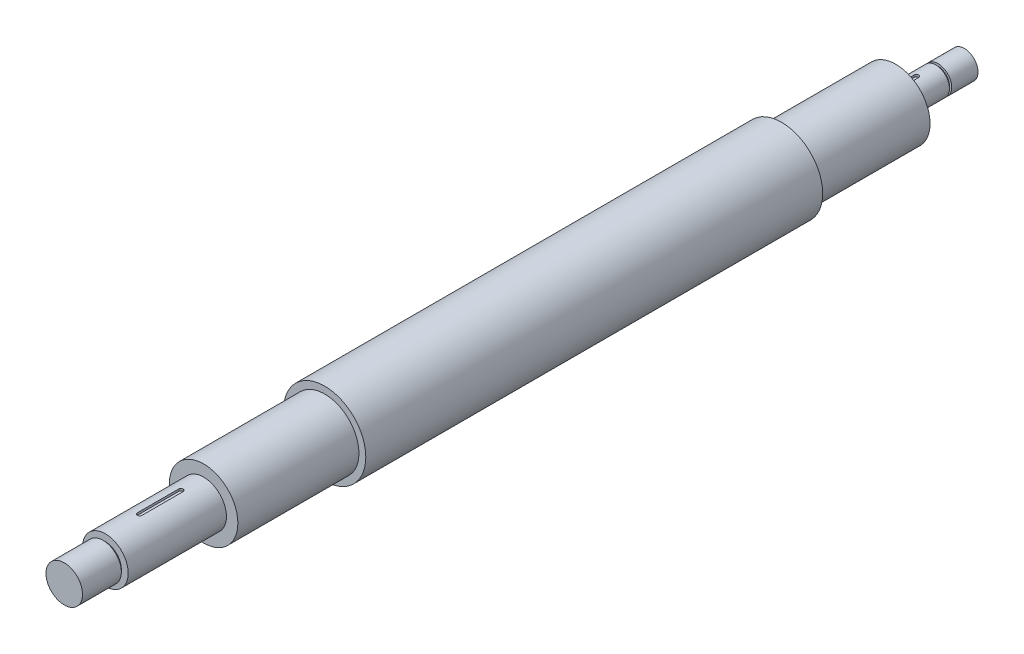
from build123d import *

# Parameters (mm, degrees)
SKETCH1_R           = 15
BOSS_EXTRUDE1_DEPTH = 50
SKETCH2_R           = 18
BOSS_EXTRUDE2_DEPTH = 200
SKETCH3_R           = 15
BOSS_EXTRUDE3_DEPTH = 53
SKETCH4_R           = 6
BOSS_EXTRUDE4_DEPTH = 30
CUT_EXTRUDE1_START  = 5
CUT_EXTRUDE1_DEPTH  = 10
CUT_EXTRUDE3_START  = -12.5
SKETCH6_R           = 6
SKETCH6_R_2         = 5
CUT_EXTRUDE3_DEPTH  = 1
SKETCH7_R           = 10
BOSS_EXTRUDE5_DEPTH = 43
CUT_EXTRUDE4_START  = 4
CUT_EXTRUDE4_DEPTH  = 12
SKETCH8_R           = 8
BOSS_EXTRUDE6_DEPTH = 18
CUT_EXTRUDE6_START  = -18
SKETCH10_R          = 9
SKETCH10_R_2        = 7
CUT_EXTRUDE6_DEPTH  = 1


with BuildPart() as part:
    # Sketch1 → Boss-Extrude1 (new body)
    with BuildSketch(Plane.XY):
        Circle(SKETCH1_R)
    extrude(amount=BOSS_EXTRUDE1_DEPTH)

    # Sketch2 → Boss-Extrude2 (add)
    with BuildSketch(Plane.XY.offset(50)):
        Circle(SKETCH2_R)
    extrude(amount=BOSS_EXTRUDE2_DEPTH)

    # Sketch3 → Boss-Extrude3 (add)
    with BuildSketch(Plane.XY.offset(250)):
        Circle(SKETCH3_R)
    extrude(amount=BOSS_EXTRUDE3_DEPTH)

    # Sketch4 → Boss-Extrude4 (add)
    with BuildSketch(Plane(origin=(0, 0, 0), x_dir=(-1, 0, 0), z_dir=(0, 0, -1))):
        with Locations(Location((0, 0, 0), (0, 0, 180))):
            Circle(SKETCH4_R)
    extrude(amount=BOSS_EXTRUDE4_DEPTH)

    # Sketch5 → Cut-Extrude1 (cut)
    with BuildSketch(Plane(origin=(0, 0, 0), x_dir=(1, 0, 0), z_dir=(0, 1, 0)).offset(CUT_EXTRUDE1_START)):
        with BuildLine():
            ThreePointArc((-1, 9), (0, 8), (1, 9))
            Line((1, 9), (-1, 9))
        make_face()
        with BuildLine():
            Line((-1, 9), (1, 9))
            ThreePointArc((1, 9), (0, 10), (-1, 9))
        make_face()
        with BuildLine():
            Line((1, 5), (1, 9))
            ThreePointArc((1, 9), (0, 8), (-1, 9))
            Line((-1, 9), (-1, 5))
            ThreePointArc((-1, 5), (0, 6), (1, 5))
        make_face()
        with BuildLine():
            ThreePointArc((-1, 5), (0, 4), (1, 5))
            Line((1, 5), (-1, 5))
        make_face()
        with BuildLine():
            Line((-1, 5), (1, 5))
            ThreePointArc((1, 5), (0, 6), (-1, 5))
        make_face()
    extrude(amount=CUT_EXTRUDE1_DEPTH, mode=Mode.SUBTRACT)

    # Sketch6 → Cut-Extrude3 (cut)
    with BuildSketch(Plane(origin=(0, 0, -30), x_dir=(-1, 0, 0), z_dir=(0, 0, -1)).offset(CUT_EXTRUDE3_START)):
        with Locations(Location((0, 0, 0), (0, 0, 180))):
            Circle(SKETCH6_R)
        Circle(SKETCH6_R_2, mode=Mode.SUBTRACT)
    extrude(amount=CUT_EXTRUDE3_DEPTH, mode=Mode.SUBTRACT)

    # Sketch7 → Boss-Extrude5 (add)
    with BuildSketch(Plane.XY.offset(303)):
        Circle(SKETCH7_R)
    extrude(amount=BOSS_EXTRUDE5_DEPTH)

    # Sketch9 → Cut-Extrude4 (cut)
    with BuildSketch(Plane(origin=(0, 5, 0), x_dir=(1, 0, 0), z_dir=(0, 1, 0)).offset(CUT_EXTRUDE4_START)):
        with BuildLine():
            ThreePointArc((1, -313), (0, -314), (-1, -313))
            Line((-1, -313), (-1, -331))
            ThreePointArc((-1, -331), (0, -330), (1, -331))
            Line((1, -331), (1, -313))
        make_face()
        with BuildLine():
            ThreePointArc((1, -331), (0, -330), (-1, -331))
            Line((-1, -331), (1, -331))
        make_face()
        with BuildLine():
            Line((1, -331), (-1, -331))
            ThreePointArc((-1, -331), (0, -332), (1, -331))
        make_face()
        with BuildLine():
            ThreePointArc((1, -313), (0, -312), (-1, -313))
            Line((-1, -313), (1, -313))
        make_face()
        with BuildLine():
            Line((1, -313), (-1, -313))
            ThreePointArc((-1, -313), (0, -314), (1, -313))
        make_face()
    extrude(amount=CUT_EXTRUDE4_DEPTH, mode=Mode.SUBTRACT)

    # Sketch8 → Boss-Extrude6 (add)
    with BuildSketch(Plane.XY.offset(346)):
        Circle(SKETCH8_R)
    extrude(amount=BOSS_EXTRUDE6_DEPTH)

    # Sketch10 → Cut-Extrude6 (cut)
    with BuildSketch(Plane.XY.offset(364).offset(CUT_EXTRUDE6_START)):
        Circle(SKETCH10_R)
        Circle(SKETCH10_R_2, mode=Mode.SUBTRACT)
    extrude(amount=CUT_EXTRUDE6_DEPTH, mode=Mode.SUBTRACT)


solid = part.part
